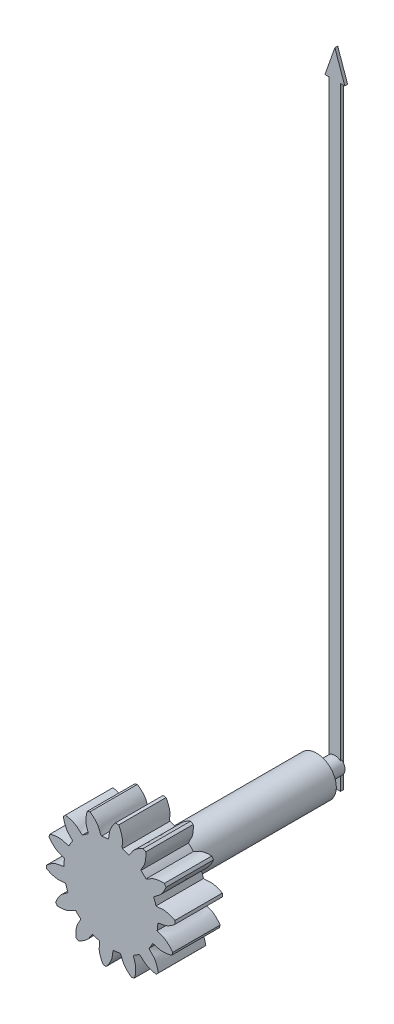
from build123d import *

# Parameters (mm, degrees)
SKETCH1_R                = 1.188
SKETCH1_R_2              = 0.5
BOSS_EXTRUDE1_DEPTH      = 1.2
BOSS_EXTRUDE2_DEPTH      = 1.2
CIRPATTERN1_COUNT        = 14
BOSS_EXTRUDE3_DEPTH      = 4
BOSS_EXTRUDE3_DEPTH_BACK = 1.2
SKETCH3_R                = 0.5
SKETCH4_R                = 0.219359104
BOSS_EXTRUDE4_DEPTH      = 0.5
BOSS_EXTRUDE5_DEPTH      = 15
BOSS_EXTRUDE5_DEPTH_BACK = 0.5
SKETCH5_W                = 0.284383346
SKETCH5_H                = 0.072697092
BOSS_EXTRUDE6_DEPTH      = 0.072697092


with BuildPart() as part:
    # Sketch1 → Boss-Extrude1 (new body)
    with BuildSketch(Plane.XY):
        Circle(SKETCH1_R)
        Circle(SKETCH1_R_2, mode=Mode.SUBTRACT)
    extrude(amount=BOSS_EXTRUDE1_DEPTH)

    # Sketch2 → Boss-Extrude2 (add)
    with BuildSketch(Plane.XY):
        with BuildLine():
            ThreePointArc((1.619448512, 0.245826193), (1.624786484, 0.207636419), (1.629223993, 0.169331571))
            add(Edge.make_bspline(
                [(1.629223993, 0.169331571), (1.591300465, 0.134739741), (1.531615848, 0.087628678), (1.445515367, 0.039548212), (1.341528029, -0.00593525), (1.248784579, -0.003185884), (1.187683187, -0.027434427)],
                knots=[0, 0, 0, 0, 0.313167223, 0.460102943, 0.600582887, 1, 1, 1, 1], degree=3))
            ThreePointArc((1.187683187, -0.027434427), (1.178416571, 0.150593446), (1.14261508, 0.325230348))
            add(Edge.make_bspline(
                [(1.619448512, 0.245826193), (1.574044618, 0.269769358), (1.504430652, 0.300356961), (1.409005971, 0.325239773), (1.296922361, 0.34311087), (1.207850842, 0.317126815), (1.14261508, 0.325230348)],
                knots=[0, 0, 0, 0, 0.313167223, 0.460102943, 0.600582887, 1, 1, 1, 1], degree=3))
        make_face()
    boss_extrude2 = extrude(amount=BOSS_EXTRUDE2_DEPTH)

    # CirPattern1: Boss-Extrude2 ×14 about axis
    cirpattern1_axis = Axis((0, 0, 1.2), (0, 0, -1))
    for i in range(1, CIRPATTERN1_COUNT):
        add(boss_extrude2.rotate(cirpattern1_axis, i * 360 / CIRPATTERN1_COUNT))

    # Sketch3 → Boss-Extrude3 (add, two sides: drawn at the far end of the back side and taken through both)
    with BuildSketch(Plane(origin=(0, 0, 0), x_dir=(-1, 0, 0), z_dir=(0, 0, -1)).offset(-BOSS_EXTRUDE3_DEPTH_BACK)):
        Circle(SKETCH3_R)
    extrude(amount=BOSS_EXTRUDE3_DEPTH + BOSS_EXTRUDE3_DEPTH_BACK)

    # Sketch4 → Boss-Extrude4 (add)
    with BuildSketch(Plane(origin=(0, 0, -4), x_dir=(-1, 0, 0), z_dir=(0, 0, -1))):
        Circle(SKETCH4_R)
    extrude(amount=BOSS_EXTRUDE4_DEPTH)

    # Sketch5 → Boss-Extrude5 (add, two sides: drawn at the far end of the back side and taken through both)
    with BuildSketch(Plane(origin=(0, 0, 0), x_dir=(1, 0, 0), z_dir=(0, 1, 0)).offset(-BOSS_EXTRUDE5_DEPTH_BACK)):
        with Locations((0, 4.5)):
            Rectangle(SKETCH5_W, SKETCH5_H)
    extrude(amount=BOSS_EXTRUDE5_DEPTH + BOSS_EXTRUDE5_DEPTH_BACK)

    # Sketch6 → Boss-Extrude6 (add)
    with BuildSketch(Plane(origin=(0, 0, -4.536348546), x_dir=(-1, 0, 0), z_dir=(0, 0, -1))):
        Polygon((0, 15), (-0.25, 15), (0, 15.713005465), (0.25, 15), align=None)
    extrude(amount=-BOSS_EXTRUDE6_DEPTH)


solid = part.part
